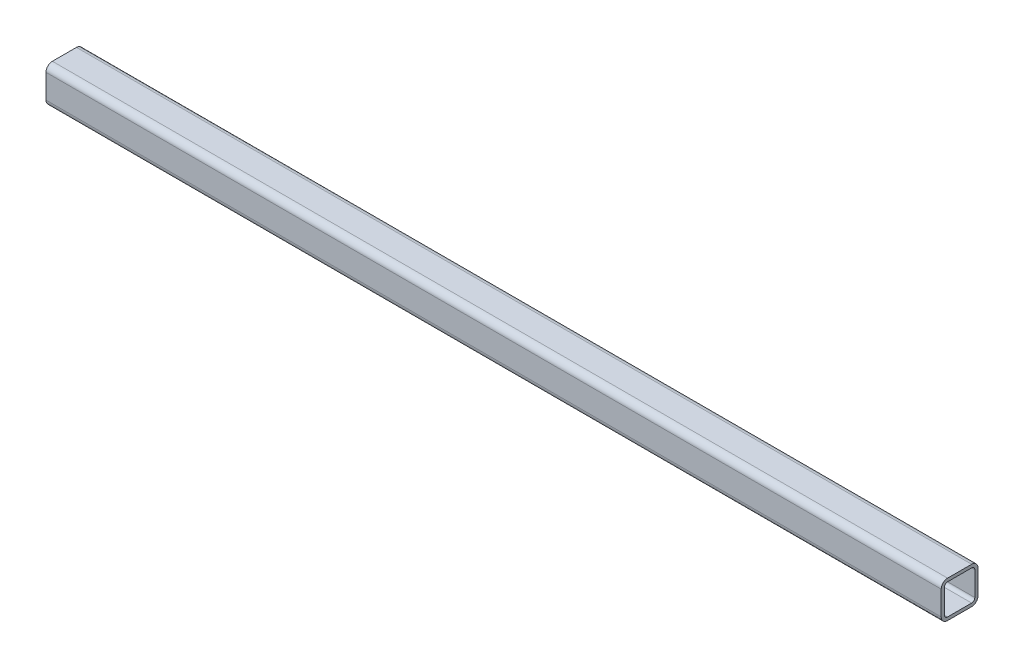
SolidWorks part; units mm, degrees
ref_plane "前视基准面" through (0, 0, 0) normal (0, 0, 1) x (1, 0, 0)
ref_plane "上视基准面" through (0, 0, 0) normal (0, 1, 0) x (1, 0, 0)
ref_plane "右视基准面" through (0, 0, 0) normal (1, 0, 0) x (0, 0, -1)
sketch3d "3D草图1"
  line L0 (0, 0, 0) -> (730, 0, 0)
  dimension "D1" = 730
other "结构构件1"
ref_plane "基准面1" through (0, 0, 0) normal (1, 0, 0) x (0, 0, -1)
sketch "Sketch1" plane through (0, 0, 0) normal (1, 0, 0) x (0, 0, -1)
  line L0 (-9.8, -12.4) -> (9.8, -12.4)
  line L1 (-12.4, -9.8) -> (-12.4, 9.8)
  line L2 (9.8, 12.4) -> (-9.8, 12.4)
  line L3 (12.4, 9.8) -> (12.4, -9.8)
  line L4 (-9.8, -15) -> (9.8, -15)
  line L5 (-15, -9.8) -> (-15, 9.8)
  line L6 (9.8, 15) -> (-9.8, 15)
  line L7 (15, 9.8) -> (15, -9.8)
  arc A0 (15, 9.8) -> (9.8, 15) centre (9.8, 9.8) ccw
  arc A1 (9.8, -15) -> (15, -9.8) centre (9.8, -9.8) ccw
  arc A2 (-15, -9.8) -> (-9.8, -15) centre (-9.8, -9.8) ccw
  arc A3 (-9.8, 15) -> (-15, 9.8) centre (-9.8, 9.8) ccw
  arc A4 (-9.8, 12.4) -> (-12.4, 9.8) centre (-9.8, 9.8) ccw
  arc A5 (12.4, 9.8) -> (9.8, 12.4) centre (9.8, 9.8) ccw
  arc A6 (9.8, -12.4) -> (12.4, -9.8) centre (9.8, -9.8) ccw
  arc A7 (-12.4, -9.8) -> (-9.8, -12.4) centre (-9.8, -9.8) ccw
  point P0 (-15, 0)
  point P1 (15, 0)
  point P2 (0, 15)
  point P3 (0, -15)
  point P4 (0, 0)
  point P5 (-15, -15)
  point P6 (15, -15)
  point P7 (15, 15)
  point P8 (-15, 15)
  point P33 (0, 0)
  dimension "D1" = 5.2
  dimension "Thickness" = 2.6
  dimension "V_leg" = 30
